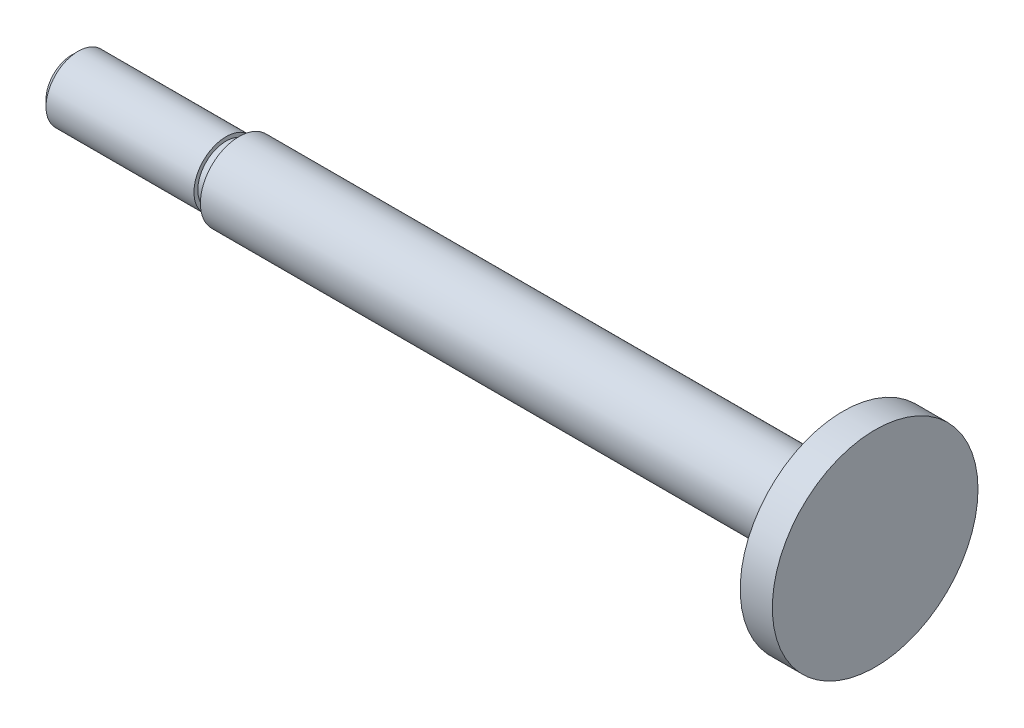
from build123d import *

# Parameters (mm, degrees)
SKETCH2_W = 1
SKETCH2_H = 2.2


with BuildPart() as part:
    # Sketch1 → Revolve1 (revolve)
    with BuildSketch(Plane.XY, mode=Mode.PRIVATE) as revolve1_sk:
        Polygon((-11, 0), (-11, 3), (36, 3), (36, 8), (38.5, 8), (38.5, 0), align=None)
    revolve(revolve1_sk.sketch.rotate(Axis((38.5, 0, 0), (-1, 0, 0)), 90), axis=Axis((38.5, 0, 0), (-1, 0, 0)))

    # Sketch2 → Revolve2 (revolve)
    with BuildSketch(Plane.XY, mode=Mode.PRIVATE) as revolve2_sk:
        with Locations((-11.5, 1.1)):
            Rectangle(SKETCH2_W, SKETCH2_H)
    revolve(revolve2_sk.sketch.rotate(Axis((-11, 0, 0), (-1, 0, 0)), 90), axis=Axis((-11, 0, 0), (-1, 0, 0)))

    # Sketch3 → Revolve3 (revolve)
    with BuildSketch(Plane.XY, mode=Mode.PRIVATE) as revolve3_sk:
        Polygon((-24, 0), (-24, 2.0095), (-23.5095, 2.5), (-12, 2.5), (-12, 0), align=None)
    revolve(revolve3_sk.sketch.rotate(Axis((-12, 0, 0), (-1, 0, 0)), 90), axis=Axis((-12, 0, 0), (-1, 0, 0)))


solid = part.part
